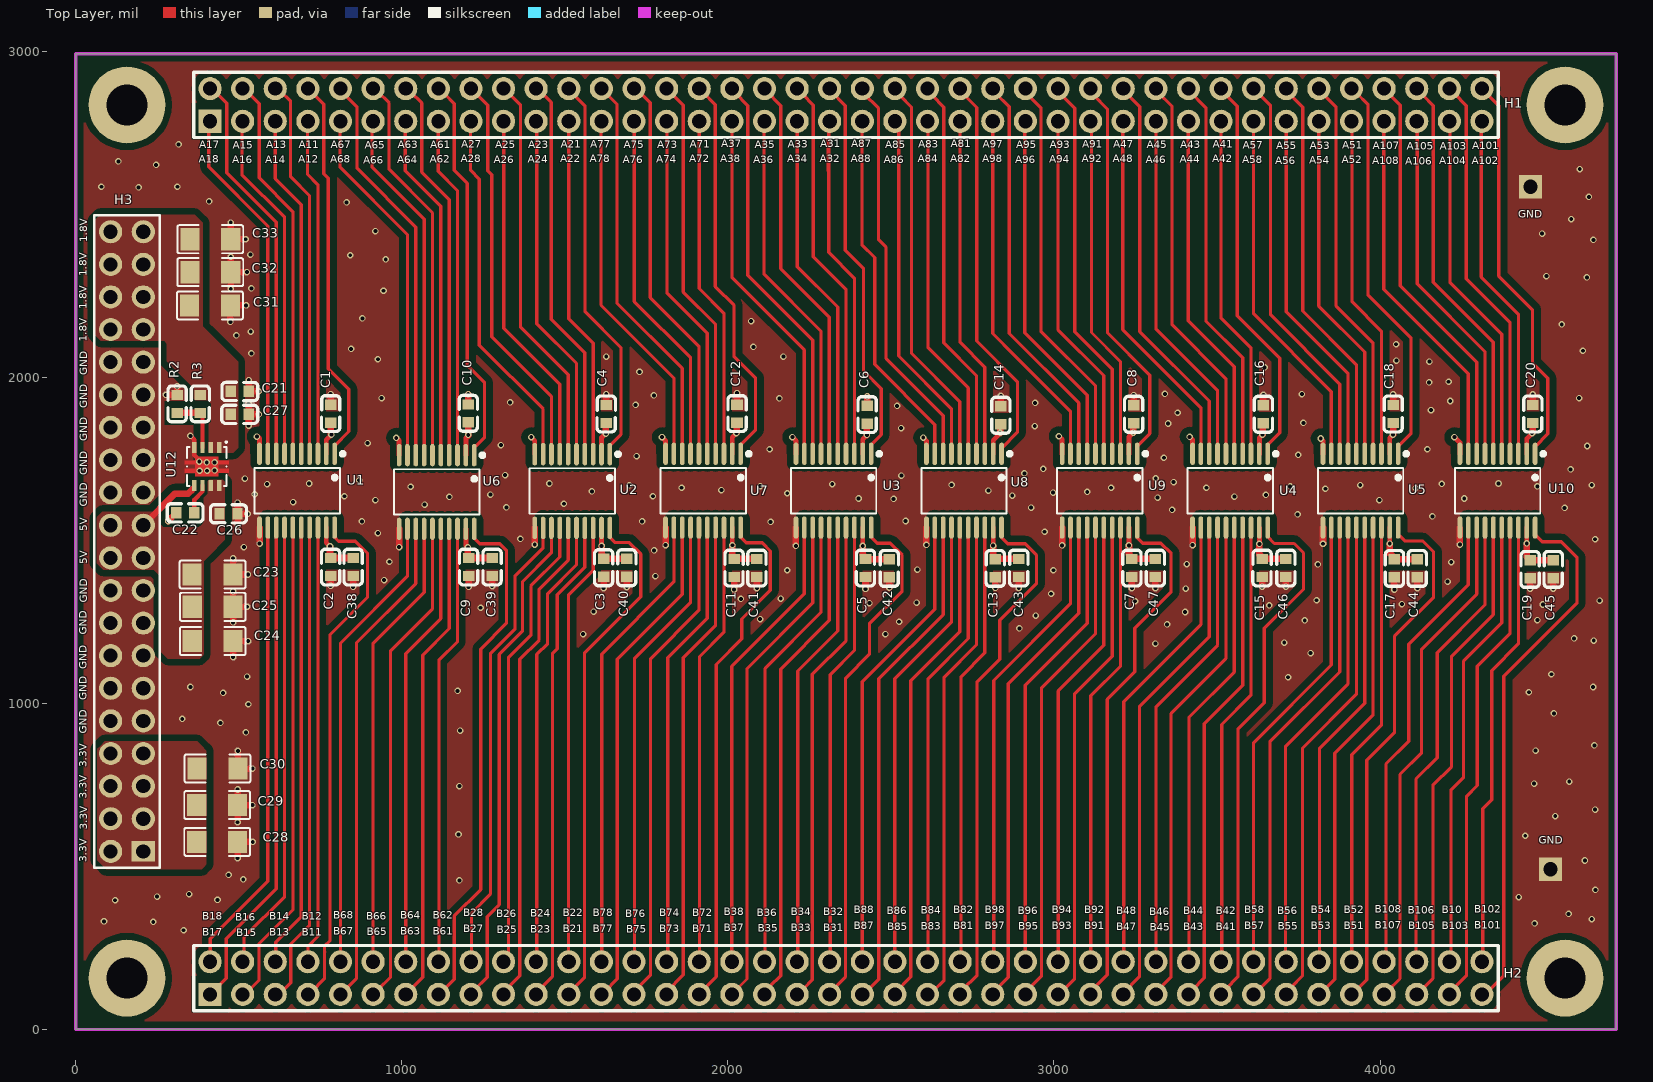
[diagram p0: Top Layer view]
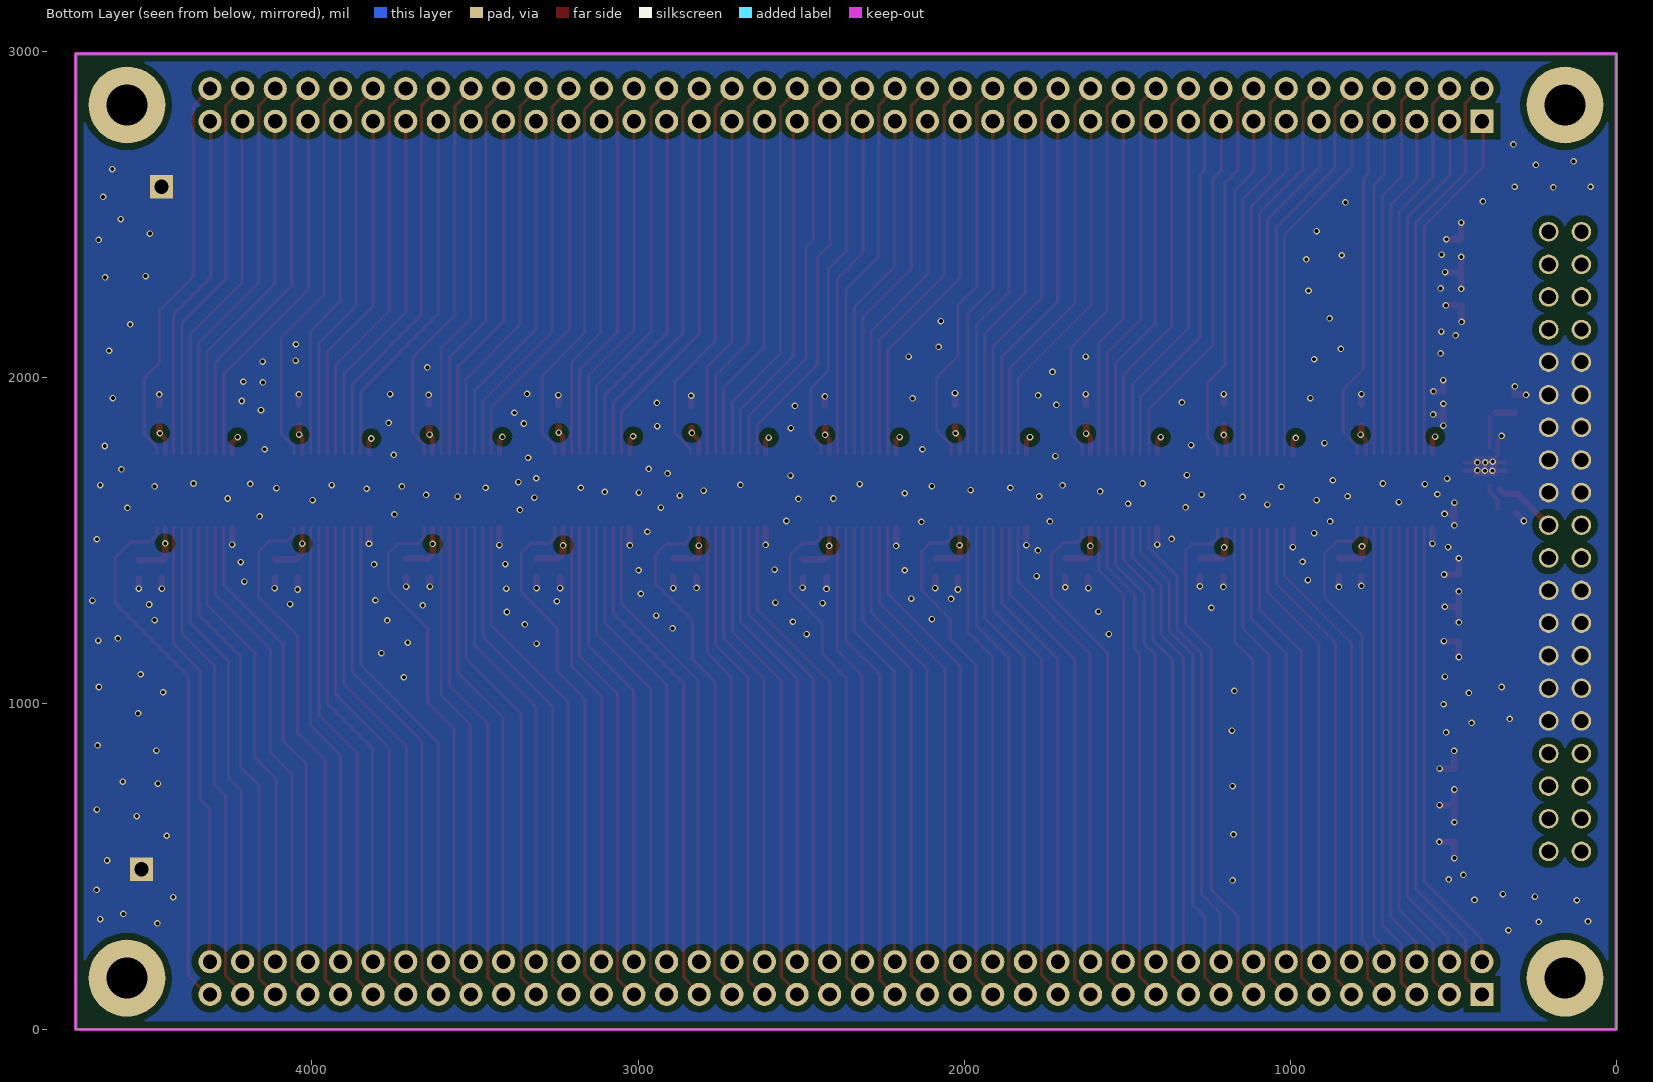
[diagram p1: Bottom Layer view, seen from below]
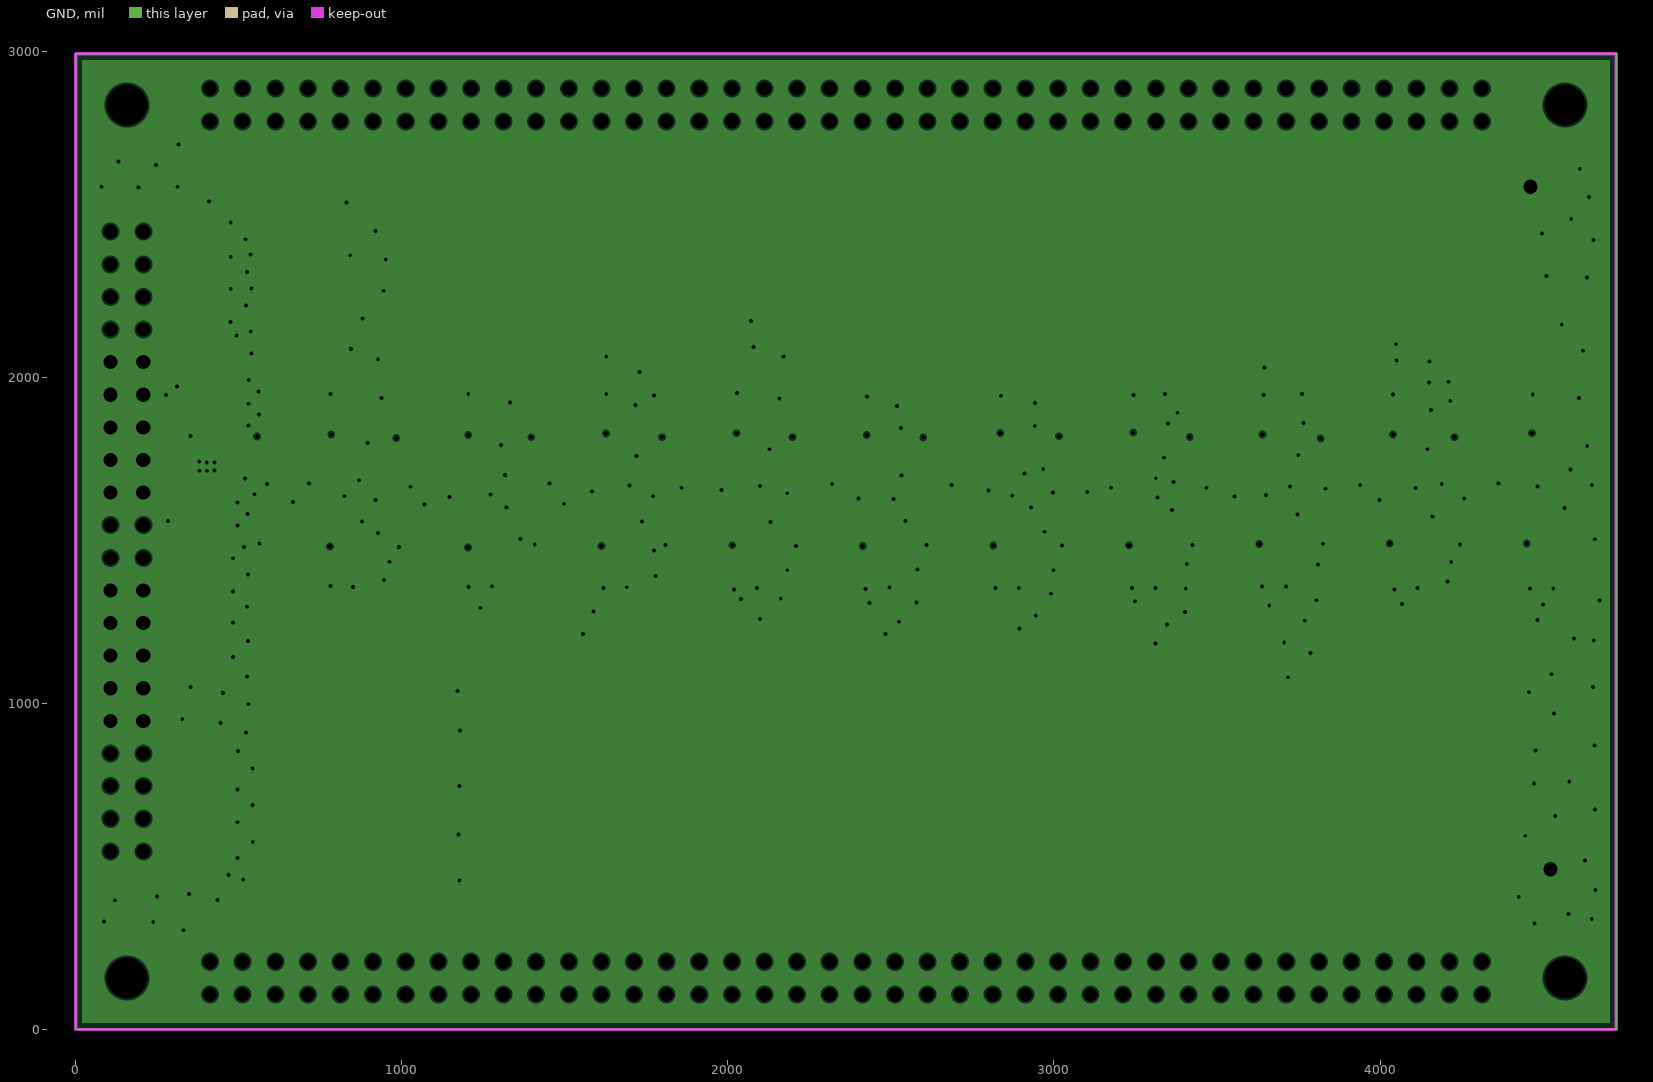
[diagram p2: GND, clearances drawn from the general rule]
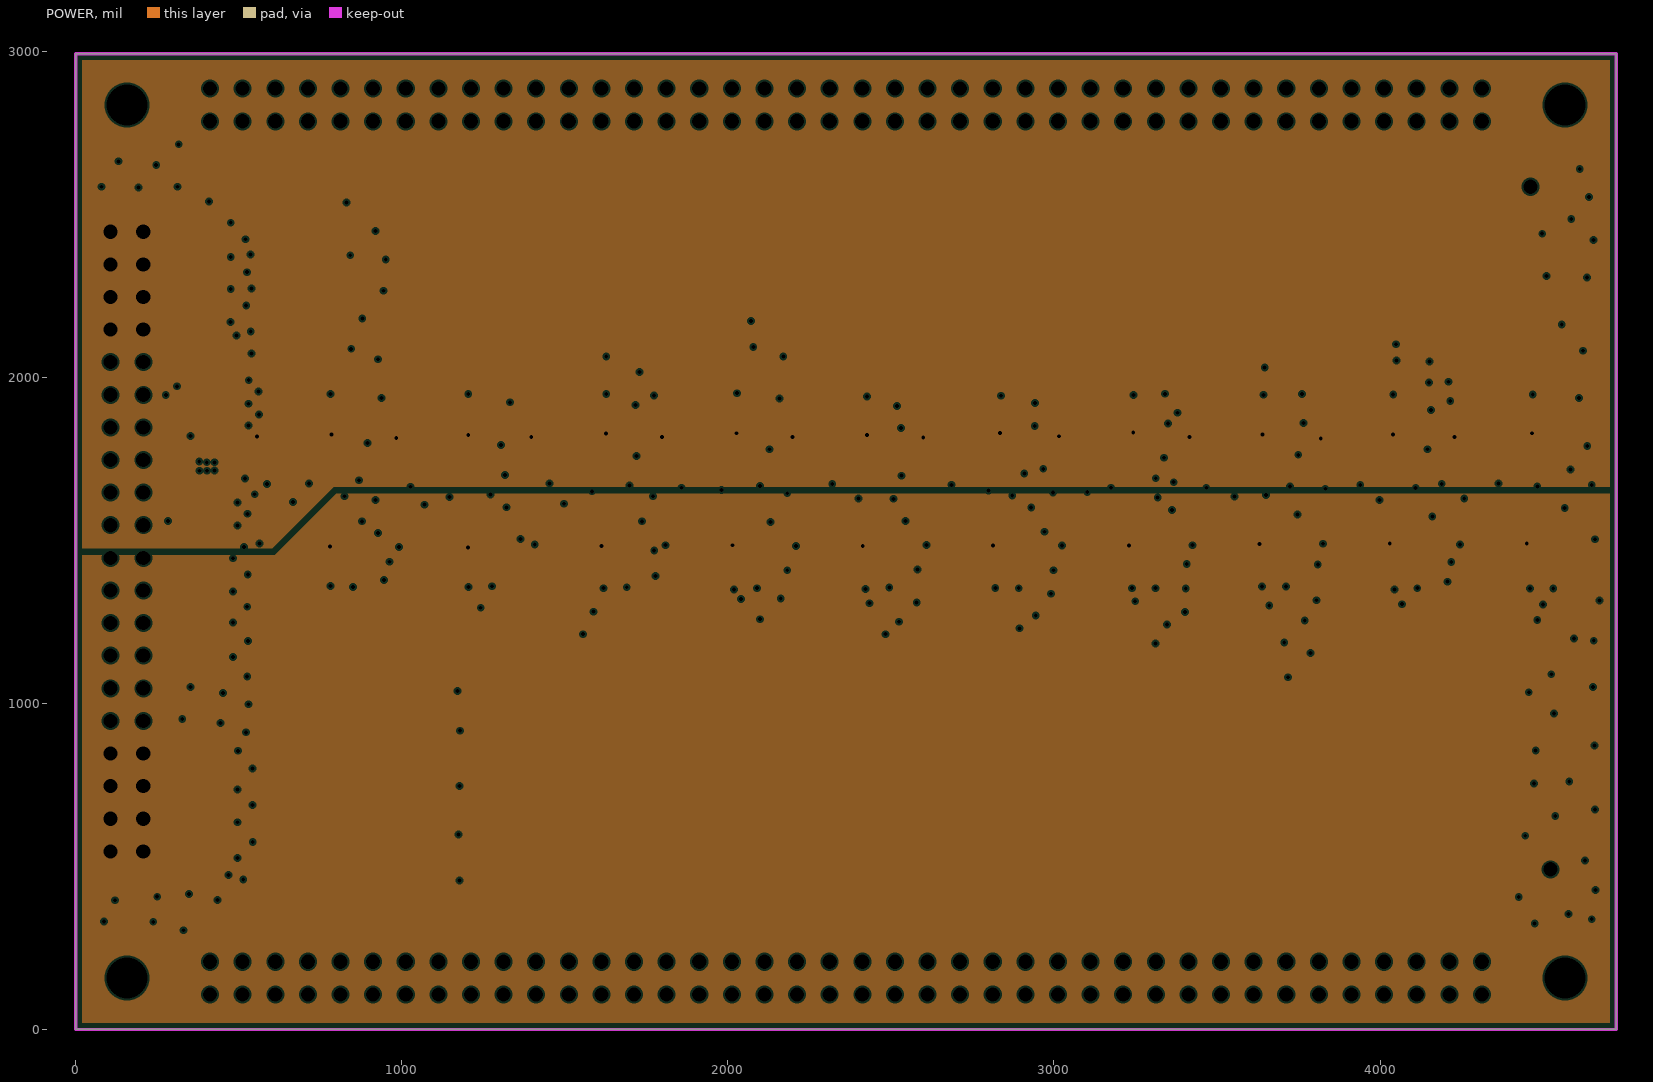
[diagram p3: POWER, clearances drawn from the general rule]
# Altium PCB MISC79033.pcbdoc (part 1 of 2)
Units mil, origin at the board's own origin, x right, y up, seen from the top; angles counter-clockwise.
Board outline 4724.41 x 2992.13 mil, 4 copper layers (Top Layer, GND, POWER, Bottom Layer); 59 components, 166 nets, 504 pads, 319 vias.

## Layer stack, top to bottom (the 12.6 mil dielectric is the usual default, probably not edited)
Top Layer: signal copper 1.4
Dielectric: core 12.6, FR-4, Dk 4.8
GND: plane copper 1.4, net GND
Dielectric: prepreg 12.6, FR-4, Dk 4.8
POWER: plane copper 1.4, net 3.3V
Dielectric: core 12.6, FR-4, Dk 4.8
Bottom Layer: signal copper 1.4

## Board outline
0,0 4724.41,0 4724.41,2992.13 0,2992.13

## Design rules (kind name [scope] priority, off if disabled: settings)
Clearance Clearance_1 [inpolygon] p1: gap=6
Clearance [All] p2: gap=6
HoleSize [All] p1: absolutevalues=TRUE maxlimit=500 minlimit=1 maxpercent=80.000 minpercent=20.000
HoleToHoleClearance [All] p1: gap=0 allowstackedmicrovias=TRUE
MinimumSolderMaskSliver [All] p1: minsoldermaskwidth=0
PlaneClearance [All] p1: clearance=6
PlaneConnect [All] p1: planeconnectstyle=Direct reliefexpansion=20 reliefentries=4 reliefconductorwidth=10 reliefairgap=10
PolygonConnect [All] p1: connectstyle=Direct reliefconductorwidth=10 reliefentries=4 polygonreliefangle="90 Angle"
RoutingVias [All] p1: holewidth=12 width=20 viastyle="Through Hole" minholewidth=12 minwidth=20 maxholewidth=12 maxwidth=20
SilkToSilkClearance [All] p1: silktosilkclearance=0
SilkscreenOverComponentPads [All] p1: minsilkscreentomaskgap=0
SolderMaskExpansion [All] p1: expansion=4
Width [All] p1: maxlimit=20 minlimit=8 preferedwidth=8 minimp=50.000000 maximp=50.000000 favimp=50.000000
21 further rules are at their usual default settings.

## Components (designator, comment, footprint, x,y, rotation, side; value= is the part's Value field where it differs from the comment)
C1 "0.1u/50V" C0603 782,1888 r270 top
C2 "0.1u/50V" C0603 782,1418 r90 top
C3 "0.1u/50V" C0603 1619,1416 r90 top
C4 "0.1u/50V" C0603 1627,1887 r270 top
C5 "0.1u/50V" C0603 2422,1415 r90 top
C6 "0.1u/50V" C0603 2427,1885 r270 top
C7 "0.1u/50V" C0603 3239,1415 r90 top
C8 "0.1u/50V" C0603 3244,1886 r270 top
C9 "0.1u/50V" C0603 1205,1418 r90 top
C10 "0.1u/50V" C0603 1204,1889 r270 top
C11 "0.1u/50V" C0603 2019,1415 r90 top
C12 "0.1u/50V" C0603 2028,1888 r270 top
C13 "0.1u/50V" C0603 2820,1414 r90 top
C14 "0.1u/50V" C0603 2837,1883 r270 top
C15 "0.1u/50V" C0603 3638,1415 r90 top
C16 "0.1u/50V" C0603 3642,1886 r270 top
C17 "0.1u/50V" C0603 4044,1414 r90 top
C18 "0.1u/50V" C0603 4040,1887 r270 top
C19 "0.1u/50V" C0603 4460,1411 r90 top
C20 "0.1u/50V" C0603 4468,1887 r270 top
C21 "4.7u/6.3v" C0603 503.26,1956.22 r180 top
C22 "10nF/50v" C0603 336,1584 r0 top
C23 "47uF/10V" C1206 420,1395 r180 top
C24 "47uF/10V" C1206 420.32,1191 r180 top
C25 "47uF/10V" C1206 420.32,1296 r180 top
C26 "1uF/50v" C0603 469,1581 r0 top
C27 "4.7u/6.3v" C0603 503,1886 r180 top
C28 "47uF/10V" C1206 434,575 r180 top
C29 "47uF/10V" C1206 434,688 r180 top
C30 "47uF/10V" C1206 435,800 r180 top
C31 "47uF/10V" C1206 411.88,2220 r180 top
C32 "47uF/10V" C1206 413,2322 r180 top
C33 "47uF/10V" C1206 413,2423 r180 top
C38 "4.7u/6.3v" C0603 851,1418 r90 top
C39 "4.7u/6.3v" C0603 1277,1418 r90 top
C40 "4.7u/6.3v" C0603 1690,1416 r90 top
C41 "4.7u/6.3v" C0603 2089,1415 r90 top
C42 "4.7u/6.3v" C0603 2495,1414 r90 top
C43 "4.7u/6.3v" C0603 2892,1415 r90 top
C44 "4.7u/6.3v" C0603 4114,1414 r90 top
C45 "4.7u/6.3v" C0603 4531,1411 r90 top
C46 "4.7u/6.3v" C0603 3711,1415 r90 top
C47 "4.7u/6.3v" C0603 3311,1415 r90 top
H1 "2.54-2*40" HDR-TH_80P-P2.54-V-M-R2-C40-S2.54 2362.2,2834.65 r0 top locked
H2 "2.54-2*40" HDR-TH_80P-P2.54-V-M-R2-C40-S2.54 2362.2,157.48 r0 top
H3 "B-2100S40P-B110" HDR-TH_40P-P2.54-V-M-R2-C20-S2.54 157.48,1496.06 r90 top locked
R2 "10k 1%" R0603 311,1918 r270 top
R3 "12.5k 1%" R0603 382,1918 r270 top
U1 "TXS0108EQPWRQ1" TSSOP-20_L6.5-W4.4-P0.65-LS6.4-BL 679,1652 r180 top
U2 "TXS0108EQPWRQ1" TSSOP-20_L6.5-W4.4-P0.65-LS6.4-BL 1523,1651 r180 top
U3 "TXS0108EQPWRQ1" TSSOP-20_L6.5-W4.4-P0.65-LS6.4-BL 2324,1652 r180 top
U4 "TXS0108EQPWRQ1" TSSOP-20_L6.5-W4.4-P0.65-LS6.4-BL 3540,1652 r180 top
U5 "TXS0108EQPWRQ1" TSSOP-20_L6.5-W4.4-P0.65-LS6.4-BL 3940,1652 r180 top
U6 "TXS0108EQPWRQ1" TSSOP-20_L6.5-W4.4-P0.65-LS6.4-BL 1107,1648 r180 top
U7 "TXS0108EQPWRQ1" TSSOP-20_L6.5-W4.4-P0.65-LS6.4-BL 1924,1652 r180 top
U8 "TXS0108EQPWRQ1" TSSOP-20_L6.5-W4.4-P0.65-LS6.4-BL 2724,1652 r180 top
U9 "TXS0108EQPWRQ1" TSSOP-20_L6.5-W4.4-P0.65-LS6.4-BL 3140,1652 r180 top
U10 "TXS0108EQPWRQ1" TSSOP-20_L6.5-W4.4-P0.65-LS6.4-BL 4360,1652 r180 top
U12 "TPS7A8001DRBR" VSON-8_L3.0-W3.0-P0.65-TL-EP 402,1726 r270 top

## Footprints (in the part's own frame and the unit in brackets; to place one, negate y for a bottom-side part, rotate by r counter-clockwise, add the part's x,y. Pads: shape width x height; smd on the part's side, far side on the other; paste and mask are expansions set on the pad)
C0603 [mm]
  rect 0.8x0.9 smd paste+0 mask+0.051: 1(-0.7,0) 2(0.7,0)
  silkscreen extent -1.41,-0.71 1.39,0.72
C1206 [mm]
  rect 1.485x1.728 smd paste-100 mask+0.051: 1(-1.593,0) 2(1.593,0)
  silkscreen extent -2.56,-1.09 2.56,1.09
HDR-TH_40P-P2.54-V-M-R2-C20-S2.54 [mm]
  rect 1.575x1.8 / inner round 1.524 / far side round 1.524 hole 1.1: 1(-24.13,-1.27)
  round 1.8 / inner round 1.524 / far side round 1.524 hole 1.1: 2(-24.13,1.27) 3(-21.59,-1.27) 4(-21.59,1.27) 5(-19.05,-1.27) 6(-19.05,1.27) 7(-16.51,-1.27) 8(-16.51,1.27) 9(-13.97,-1.27) 10(-13.97,1.27) 11(-11.43,-1.27) 12(-11.43,1.27) 13(-8.89,-1.27) 14(-8.89,1.27) 15(-6.35,-1.27) 16(-6.35,1.27) 17(-3.81,-1.27) 18(-3.81,1.27) 19(-1.27,-1.27) 20(-1.27,1.27) 21(1.27,-1.27) 22(1.27,1.27) 23(3.81,-1.27) 24(3.81,1.27) 25(6.35,-1.27) 26(6.35,1.27) 27(8.89,-1.27) 28(8.89,1.27) 29(11.43,-1.27) 30(11.43,1.27) 31(13.97,-1.27) 32(13.97,1.27) 33(16.51,-1.27) 34(16.51,1.27) 35(19.05,-1.27) 36(19.05,1.27) 37(21.59,-1.27) 38(21.59,1.27) 39(24.13,-1.27) 40(24.13,1.27)
  silkscreen extent -25.4,-2.54 25.4,2.54
HDR-TH_80P-P2.54-V-M-R2-C40-S2.54 [mm]
  rect 1.8x1.8 hole 1.1 paste+0 mask+0.051: 1(-49.53,-1.27)
  round 1.8 hole 1.1 paste+0 mask+0.051: 2(-49.53,1.27) 3(-46.99,-1.27) 4(-46.99,1.27) 5(-44.45,-1.27) 6(-44.45,1.27) 7(-41.91,-1.27) 8(-41.91,1.27) 9(-39.37,-1.27) 10(-39.37,1.27) 11(-36.83,-1.27) 12(-36.83,1.27) 13(-34.29,-1.27) 14(-34.29,1.27) 15(-31.75,-1.27) 16(-31.75,1.27) 17(-29.21,-1.27) 18(-29.21,1.27) 19(-26.67,-1.27) 20(-26.67,1.27) 21(-24.13,-1.27) 22(-24.13,1.27) 23(-21.59,-1.27) 24(-21.59,1.27) 25(-19.05,-1.27) 26(-19.05,1.27) 27(-16.51,-1.27) 28(-16.51,1.27) 29(-13.97,-1.27) 30(-13.97,1.27) 31(-11.43,-1.27) 32(-11.43,1.27) 33(-8.89,-1.27) 34(-8.89,1.27) 35(-6.35,-1.27) 36(-6.35,1.27) 37(-3.81,-1.27) 38(-3.81,1.27) 39(-1.27,-1.27) 40(-1.27,1.27) 41(1.27,-1.27) 42(1.27,1.27) 43(3.81,-1.27) 44(3.81,1.27) 45(6.35,-1.27) 46(6.35,1.27) 47(8.89,-1.27) 48(8.89,1.27) 49(11.43,-1.27) 50(11.43,1.27) 51(13.97,-1.27) 52(13.97,1.27) 53(16.51,-1.27) 54(16.51,1.27) 55(19.05,-1.27) 56(19.05,1.27) 57(21.59,-1.27) 58(21.59,1.27) 59(24.13,-1.27) 60(24.13,1.27) 61(26.67,-1.27) 62(26.67,1.27) 63(29.21,-1.27) 64(29.21,1.27) 65(31.75,-1.27) 66(31.75,1.27) 67(34.29,-1.27) 68(34.29,1.27) 69(36.83,-1.27) 70(36.83,1.27) 71(39.37,-1.27) 72(39.37,1.27) 73(41.91,-1.27) 74(41.91,1.27) 75(44.45,-1.27) 76(44.45,1.27) 77(46.99,-1.27) 78(46.99,1.27) 79(49.53,-1.27) 80(49.53,1.27)
  silkscreen extent -50.8,-2.54 50.8,2.54
R0603 [mm]
  rect 0.8x0.9 smd paste+0 mask+0.051: 1(-0.7,0) 2(0.7,0)
  silkscreen extent -1.41,-0.71 1.39,0.72
TSSOP-20_L6.5-W4.4-P0.65-LS6.4-BL [mm]
  oval 0.364x1.742 smd paste+0 mask+0.051: 1(-2.925,-2.871) 2(-2.275,-2.871) 3(-1.625,-2.871) 4(-0.975,-2.871) 5(-0.325,-2.871) 6(0.325,-2.871) 7(0.975,-2.871) 8(1.625,-2.871) 9(2.275,-2.871) 10(2.925,-2.871) 11(2.925,2.871) 12(2.275,2.871) 13(1.625,2.871) 14(0.975,2.871) 15(0.325,2.871) 16(-0.325,2.871) 17(-0.975,2.871) 18(-1.625,2.871) 19(-2.275,2.871) 20(-2.925,2.871)
  silkscreen extent -3.71,-3.02 3.33,1.77
VSON-8_L3.0-W3.0-P0.65-TL-EP [mm]
  rect 0.85x0.34 smd paste+0 mask+0.051: 1(-1.476,0.975) 2(-1.476,0.325) 3(-1.476,-0.325) 4(-1.476,-0.975) 5(1.476,-0.975) 6(1.476,-0.325) 7(1.476,0.325) 8(1.476,0.975)
  Top Layer region: -0.76,0.89 -0.47,0.89 -0.47,1.71 -0.18,1.71 -0.18,0.88 0.18,0.88 0.18,1.71 0.47,1.71 0.47,0.88 0.76,0.88 0.76,-0.89 0.47,-0.89 0.47,-1.71 0.18,-1.71 0.18,-0.89 -0.18,-0.89 -0.18,-1.71 -0.47,-1.71 -0.47,-0.89 -0.76,-0.89 -0.76,0.89
  silkscreen extent -1.96,-1.52 1.52,1.58

## Part data
C1 C2 C3 C4 C5 C6 C7 C8 C9 C10 C11 C12 C13 C14 C15 C16 C17 C18 C19 C20: library part 0.1u
C21 C27 C38 C39 C40 C41 C42 C43 C44 C45 C46 C47: library part 4.7u
C22: library part 10nF
C23 C24 C25 C28 C29 C30 C31 C32 C33: library part 4.7uF
C26: library part 1uF

## Free pads (board coordinates)
  round 236.22 hole 125.98: 0(157.48,157.48) 0(157.48,2834.65) 0(4566.93,157.48) 0(4566.93,2834.65)
  rect 70.87x70.87 hole 43.31: 1(4461,2584) 1(4523,491)

## Via types
v1: diameter 20, hole 12, Top Layer to Bottom Layer, 319 vias

## Nets (pads, with @x,y where several pads share a name; then routed paths per layer and width w, separated by ;. In a path a pad name is that pad's centre, name@x,y a point inside that pad or via, vN(x,y) a via of type N, cw(c..) or ccw(c..) an arc to the next point about the centre after c; other vN are vias at no path point)
1.8V: C1.2 C4.2 C6.2 C8.2 C10.2 C12.2 C14.2 C16.2 C18.2 C20.2 C21.2 C27.2 C31.2 C32.2 C33.2 H3.33 H3.34 H3.35 H3.36 H3.37 H3.38 H3.39 H3.40 R3.1 U1.2 U1.10 U2.2 U2.10 U3.2 U3.10 U4.2 U4.10 U5.2 U5.10 U6.2 U6.10 U7.2 U7.10 U8.2 U8.10 U9.2 U9.10 U10.2 U10.10 U12.1 U12.2 | length 1477.9
  Top Layer w13: v1@555,1820 v1@557.5,1817.5 ; v1@783,1825 v1(784,1824)
  Top Layer w14: v1@984,1813 985,1812 v1@985.5,1811.5
  Top Layer w15: v1(556,1818) 558,1818 563.84,1812.16 U1.10@563.84,1765.03 ; U1.2@768.57,1765.03 768.57,1807.57 v1@785,1824 ; v1(983,1814) v1@984,1813 ; v1@986,1812 991.84,1806.16 U6.10@991.84,1761.03 ; U6.2@1196.57,1761.03 1196.57,1813.57 1204,1821 v1(1204,1823) ; v1(1397,1816) 1407.84,1805.16 U2.10@1407.84,1764.03 ; U2.2@1612.57,1764.03 1612.57,1814.57 1626,1828 v1(1626,1827) ; v1(1798,1816) 1808.84,1805.16 U7.10@1808.84,1765.03 ; U7.2@2013.57,1765.03 2013.57,1815.57 2027,1829 v1(2026,1828) ; v1(2198,1816) 2208.84,1805.16 U3.10@2208.84,1765.03 ; U3.2@2413.57,1765.03 2413.57,1809.57 2426,1822 v1(2426,1823) ; v1(2599,1815) 2608.84,1805.16 U8.10@2608.84,1765.03 ; U8.2@2813.57,1765.03 2813.57,1806.57 2835,1828 v1(2835,1829) ; v1(3015,1819) 3024.84,1809.16 U9.10@3024.84,1765.03 ; U9.2@3229.57,1765.03 3229.57,1816.57 v1(3243,1830) ; v1(3416,1817) 3424.84,1808.16 U4.10@3424.84,1765.03 ; U4.2@3629.57,1765.03 3629.57,1813.57 3640,1824 v1(3639,1824) ; v1(3818,1812) 3824.84,1805.16 U5.10@3824.84,1765.03 ; U5.2@4029.57,1765.03 4029.57,1813.57 4040,1824 v1(4039,1824) ; v1(4228,1816) 4244.84,1799.16 U10.10@4244.84,1765.03 ; U10.2@4449.57,1765.03 4449.57,1811.57 4468,1830 v1(4466,1828)
  Top Layer w20: v1@783,1825 C1.2@783,1851 ; v1@1204,1821 C10.2@1204,1853 ; v1@1626,1828 C4.2@1626,1851 ; v1@2027,1829 C12.2@2027,1849 ; v1@2426,1822 C6.2@2426,1847 ; v1@2835,1828 C14.2@2835,1845 ; v1(3243,1830) C8.2@3243,1849 ; v1@3640,1824 C16.2@3640,1847 ; v1@4040,1824 C18.2@4040,1853 ; v1@4468,1830 C20.2@4468,1849
3.3V: C2.2 C3.2 C5.2 C7.2 C9.2 C11.2 C13.2 C15.2 C17.2 C19.2 C28.2 C29.2 C30.2 C38.2 C39.2 C40.2 C41.2 C42.2 C43.2 C44.2 C45.2 C46.2 C47.2 H3.1 H3.2 H3.3 H3.4 H3.5 H3.6 H3.7 H3.8 U1.19 U2.19 U3.19 U4.19 U5.19 U6.19 U7.19 U8.19 U9.19 U10.19 | length 1685.5
  Top Layer w15: U1.19@768.57,1538.97 768.57,1492.43 v1(780,1481) ; U6.19@1196.57,1534.97 1196.57,1484.43 v1(1203,1478) ; v1(1612.57,1482.43) U2.19@1612.57,1537.97 ; v1(2013.57,1484.57) U7.19@2013.57,1538.97 ; v1(2413.57,1482.57) U3.19@2413.57,1538.97 ; v1(2813.57,1483.43) U8.19@2813.57,1538.97 ; v1(3229.57,1484.43) U9.19@3229.57,1538.97 ; v1(3629.57,1488.57) U4.19@3629.57,1538.97 ; v1(4029.57,1489.57) U5.19@4029.57,1538.97 ; v1(4449.57,1490.43) U10.19@4449.57,1538.97
  Top Layer w20: v1@780,1479 780,1449.11 783.55,1445.55 C38.2@851,1445.55 ; v1@1202,1478 1202,1451 1207.45,1445.55 C39.2@1277,1445.55 ; v1@1613,1483 1613,1456 1625.45,1443.55 C40.2@1690,1443.55 ; v1@2014,1485 2014,1450.11 2021.55,1442.55 C41.2@2089,1442.55 ; v1@2414,1482 2414,1455 2427.45,1441.55 C42.2@2495,1441.55 ; v1@2814,1482 2814,1449 2820.44,1442.55 C43.2@2892,1442.55 ; v1@3230,1484 3230,1457 3244.44,1442.55 C47.2@3311,1442.55 ; v1@3630,1487 3630,1456 3643.44,1442.55 C46.2@3711,1442.55 ; v1@4030,1489 4030,1459 4047.44,1441.55 C44.2@4114,1441.55 ; v1@4449,1488 4449,1449.55 C19.2@4460,1438.55 ; C19.2@4455.44,1438.55 C19.2@4460,1438.55 ; C45.2@4531,1438.55 C19.2@4460,1438.55
+5V: C23.2 C24.2 C25.2 C26.1 H3.19 H3.20 H3.21 H3.22 U12.5 U12.7 U12.8 | length 196.1
  Top Layer w20: H3.21@207.48,1546.06 304.42,1643 345,1643 U12.5@358,1656
A11: H1.8 U1.1 | length 1181
  Top Layer w10: H1.8@719,2879 761,2837 761,2639 761,2637 761,2624 775,2610 775,2026 837.5,1963.5 837.5,1833.5 794.16,1790.16 U1.1@794.16,1765.03
A12: H1.7 U1.3 | length 1030.2
  Top Layer w10: H1.7@711,2782 711,2622 742.98,2590.02 U1.3@742.98,1765.03
A13: H1.6 U1.4 | length 1149
  Top Layer w10: H1.6@628,2877 659,2846 659,2614 717.39,2555.61 U1.4@717.39,1765.03
A14: H1.5 U1.5 | length 1046
  Top Layer w10: H1.5@612,2778 612,2609 691.8,2529.2 U1.5@691.8,1765.03
A15: H1.4 U1.6 | length 1170.5
  Top Layer w10: H1.4@525,2877 563,2839 563,2611 666.2,2507.8 U1.6@666.2,1765.03
A16: H1.3 U1.7 | length 1062.1
  Top Layer w10: H1.3@510,2773 510,2621 640.61,2490.39 U1.7@640.61,1765.03
A17: H1.2 U1.8 | length 1180.4
  Top Layer w10: H1.2@433,2870 463,2840 463,2627 615.02,2474.98 U1.8@615.02,1765.03
A18: H1.1 U1.9 | length 1157.9
  Top Layer w10: 408,2726 408,2654 ; H1.1@410,2775 408,2773 408,2654 ; U1.9@589.43,1765.03 589.43,2463.57 408,2645 408,2654
A21: H1.24 U2.1 | length 1181.7
  Top Layer w10: H1.24@1523,2870 1562,2831 1562,2201 1672,2091 1672,1824 1638.16,1790.16 U2.1@1638.16,1764.03
A22: H1.23 U2.3 | length 1180.3
  Top Layer w10: 1512,2632 1512,2727 ; 1512,2738.21 1512,2706 ; H1.23@1517,2784 1512,2779 1512,2706 ; U2.3@1586.98,1764.03 1586.98,2104.02 1512,2179 1512,2706
A23: H1.22 U2.4 | length 1171.3
  Top Layer w10: H1.22@1423,2878 1458.64,2842.36 1458.64,2177.36 1561.39,2074.61 U2.4@1561.39,1764.03
A24: H1.21 U2.5 | length 1064.4
  Top Layer w10: 1414,2736 1414,2724 ; H1.21@1414,2766 1414,2724 ; U2.5@1535.8,1764.03 1535.8,2042.2 1414,2164 1414,2724
A25: H1.20 U2.6 | length 1183.9
  Top Layer w10: H1.20@1327,2872 1364,2835 1364,2154 1510.2,2007.8 U2.6@1510.2,1764.03
A26: H1.19 U2.7 | length 1100.1
  Top Layer w10: 1313,2736 1313,2712 ; H1.19@1313,2769 1313,2712 ; U2.7@1484.61,1764.03 1484.61,1978.39 1313,2150 1313,2712
A27: H1.18 U2.8 | length 1204.5
  Top Layer w10: H1.18@1226,2872 1264,2834 1264,2633 1276,2621 1276,2124 1459.02,1940.98 U2.8@1459.02,1764.03
A28: H1.17 U2.9 | length 1106.5
  Top Layer w10: 1211,2733 1211,2721 ; H1.17@1212,2766 1211,2765 1211,2721 ; U2.9@1433.43,1764.03 1433.43,1902.57 1238,2098 1238,2607 1211,2634 1211,2721
A31: H1.40 U3.1 | length 1187.1
  Top Layer w10: H1.40@2317,2876 2360,2833 2360,2810 2360,2389 2416,2333 2416,2019 2470,1965 2470,1824 2439.16,1793.16 U3.1@2439.16,1765.03
A32: H1.39 U3.3 | length 1142.7
  Top Layer w10: 2308,2633 2308,2728 ; 2309,2734 2309,2714 ; H1.39@2309,2760 2309,2714 ; U3.3@2387.98,1765.03 2387.98,2304.02 2309,2383 2309,2714
A33: H1.38 U3.4 | length 1157.2
  Top Layer w10: H1.38@2229,2867 2262,2834 2262,2369 2362.39,2268.61 U3.4@2362.39,1765.03
A34: H1.37 U3.5 | length 1069.7
  Top Layer w10: 2213,2736 2213,2723 ; H1.37@2214,2770 2213,2769 2213,2723 ; U3.5@2336.8,1765.03 2336.8,2215.2 2213,2339 2213,2723
A35: H1.36 U3.6 | length 1193.4
  Top Layer w10: H1.36@2117,2878 2162,2833 2162,2333 2311.2,2183.8 U3.6@2311.2,1765.03
A36: H1.35 U3.7 | length 1094.6
  Top Layer w10: 2111,2738.21 2111,2717 ; H1.35@2116,2764 2111,2759 2111,2717 ; U3.7@2285.61,1765.03 2285.61,2141.39 2111,2316 2111,2717
A37: H1.34 U3.8 | length 1205.6
  Top Layer w10: H1.34@2022,2872 2061,2833 2061,2312 2260.02,2112.98 U3.8@2260.02,1765.03
A38: H1.33 U3.9 | length 1097.7
  Top Layer w10: 2013,2727 2013,2719 ; H1.33@2013,2763 2013,2719 ; U3.9@2234.43,1765.03 2234.43,2083.57 2013,2305 2013,2719
A41: H1.64 U4.1 | length 1197.1
  Top Layer w10: H1.64@3521,2876 3521,2872 3562,2831 3562,2188 3692,2058 3692,1830 3655.16,1793.16 U4.1@3655.16,1765.03
A42: H1.63 U4.3 | length 1040.1
  Top Layer w10: 3512,2735 3512,2727 ; H1.63@3512,2759 3512,2727 ; U4.3@3603.98,1765.03 3603.98,2090.02 3512,2182 3512,2727
A43: H1.62 U4.4 | length 1185.2
  Top Layer w10: H1.62@3409,2876 3416,2876 3465.77,2826.23 3465.77,2172.23 3578.39,2059.61 U4.4@3578.39,1765.03
A44: H1.61 U4.5 | length 1061.1
  Top Layer w10: H1.61@3414,2767 3412,2765 3412,2173 3552.8,2032.2 U4.5@3552.8,1765.03
A45: H1.60 U4.6 | length 1197
  Top Layer w10: H1.60@3317,2875 3362,2830 3362,2161 3527.2,1995.8 U4.6@3527.2,1765.03
A46: H1.59 U4.7 | length 1074.1
  Top Layer w10: H1.59@3313,2761 3313,2147 3501.61,1958.39 U4.7@3501.61,1765.03
A47: H1.58 U4.8 | length 1213
  Top Layer w10: H1.58@3220,2872 3263,2829 3263,2140 3476.02,1926.98 U4.8@3476.02,1765.03
A48: H1.57 U4.9 | length 1101.4
  Top Layer w10: 3211,2738.21 3211,2731 ; H1.57@3211,2760 3211,2731 ; U4.9@3450.43,1765.03 3450.43,1906.57 3211,2146 3211,2731
A51: H1.72 U5.1 | length 1194.5
  Top Layer w10: H1.72@3926,2873 3963,2836 3963,2251 4095,2119 4095,1828 4055.16,1788.16 U5.1@4055.16,1765.03
A52: H1.71 U5.3 | length 1039.5
  Top Layer w10: 3914,2738.21 3914,2733 ; H1.71@3914,2762 3914,2733 ; U5.3@4003.98,1765.03 4003.98,2141.02 3914,2231 3914,2733
A53: H1.70 U5.4 | length 1152.4
  Top Layer w10: H1.70@3835,2858 3865,2828 3865,2218 3978.39,2104.61 U5.4@3978.39,1765.03
A54: H1.69 U5.5 | length 1059.1
  Top Layer w10: H1.69@3814,2765 3812,2763 3812,2218 3952.8,2077.2 U5.5@3952.8,1765.03
A55: H1.68 U5.6 | length 1187.6
  Top Layer w10: H1.68@3723,2868 3763,2828 3763,2203 3927.2,2038.8 U5.6@3927.2,1765.03
A56: H1.67 U5.7 | length 1076.5
  Top Layer w10: H1.67@3712,2763 3712,2200 3901.61,2010.39 U5.7@3901.61,1765.03
A57: H1.66 U5.8 | length 1209.5
  Top Layer w10: H1.66@3626,2871 3664,2833 3664,2191 3876.02,1978.98 U5.8@3876.02,1765.03
A58: H1.65 U5.9 | length 1093.7
  Top Layer w10: H1.65@3612,2760 3612,2194 3850.43,1955.57 U5.9@3850.43,1765.03
A61: H1.16 U6.1 | length 1172.1
  Top Layer w10: H1.16@1131,2869 1161,2839 1161,2810 1161,2634 1201,2594 1201,2036 1254,1983 1254,1816 1222.16,1784.16 U6.1@1222.16,1761.03
A62: H1.15 U6.3 | length 1036.2
  Top Layer w10: 1112,2733 1112,2726 ; H1.15@1114,2765 1112,2763 1112,2726 ; U6.3@1170.98,1761.03 1170.98,2572.02 1112,2631 1112,2726
A63: H1.14 U6.4 | length 1161.6
  Top Layer w10: H1.14@1028,2874 1061,2841 1061,2629 1145.39,2544.61 U6.4@1145.39,1761.03
A64: H1.13 U6.5 | length 1060
  Top Layer w10: H1.13@1011,2776 1011,2633 1119.8,2524.2 U6.5@1119.8,1761.03
A65: H1.12 U6.6 | length 1183.2
  Top Layer w10: H1.12@927,2875 961,2841 961,2637 1094.2,2503.8 U6.6@1094.2,1761.03
A66: H1.11 U6.7 | length 1069.1
  Top Layer w10: H1.11@909,2764 909,2644 1068.61,2484.39 U6.7@1068.61,1761.03
A67: H1.10 U6.8 | length 1191
  Top Layer w10: H1.10@828,2863 863,2828 863,2640 1043.02,2459.98 U6.8@1043.02,1761.03
A68: H1.9 U6.9 | length 1108.5
  Top Layer w10: H1.9@811,2784 811,2644 1017.43,2437.57 U6.9@1017.43,1761.03
A71: H1.32 U7.1 | length 1193.6
  Top Layer w10: H1.32@1924,2873 1961,2836 1961,2808 1961,2278 2019,2220 2019,2063 2085,1997 2085,1839 2039.16,1793.16 U7.1@2039.16,1765.03
A72: H1.31 U7.3 | length 1055.7
  Top Layer w10: H1.31@1907,2769 1912,2764 1912,2720 ; 1912,2738.21 1912,2720 ; U7.3@1987.98,1765.03 1987.98,2196.02 1912,2272 1912,2720
A73: H1.30 U7.4 | length 1175.2
  Top Layer w10: H1.30@1817,2880 1863,2834 1863,2261 1962.39,2161.61 U7.4@1962.39,1765.03
A74: H1.29 U7.5 | length 1077.5
  Top Layer w10: 1813,2738.21 1813,2713 ; H1.29@1813,2766 1813,2713 ; U7.5@1936.8,1765.03 1936.8,2135.2 1813,2259 1813,2713
A75: H1.28 U7.6 | length 1196.8
  Top Layer w10: H1.28@1721,2883 1762,2842 1762,2244 1911.2,2094.8 U7.6@1911.2,1765.03
A76: H1.27 U7.7 | length 1072.5
  Top Layer w10: H1.27@1713,2766 1713,2232 1885.61,2059.39 U7.7@1885.61,1765.03
A77: H1.26 U7.8 | length 1215.6
  Top Layer w10: H1.26@1617,2880 1660,2837 1660,2227 1860.02,2026.98 U7.8@1860.02,1765.03
A78: H1.25 U7.9 | length 1120.3
  Top Layer w10: 1611,2734 1611,2715 ; H1.25@1613,2773 1611,2771 1611,2715 ; U7.9@1834.43,1765.03 1834.43,1997.57 1611,2221 1611,2715
A81: H1.48 U8.1 | length 1203
  Top Layer w10: H1.48@2713,2873 2717,2873 2763,2827 2763,2111 2888,1986 2888,1831 2839.16,1782.16 U8.1@2839.16,1765.03
A82: H1.47 U8.3 | length 1041.7
  Top Layer w10: H1.47@2709,2774 2712,2771 2712,2107 2787.98,2031.02 U8.3@2787.98,1765.03
A83: H1.46 U8.4 | length 1155.5
  Top Layer w10: H1.46@2626,2864 2662,2828 2662,2105 2762.39,2004.61 U8.4@2762.39,1765.03
A84: H1.45 U8.5 | length 1058.9
  Top Layer w10: H1.45@2612,2767 2614,2765 2614,2733 ; 2614,2738.21 2614,2733 ; U8.5@2736.8,1765.03 2736.8,1967.2 2614,2090 2614,2733
A85: H1.44 U8.6 | length 1173.9
  Top Layer w10: H1.44@2528,2863 2563,2828 2563,2073 2711.2,1924.8 U8.6@2711.2,1765.03
A86: H1.43 U8.7 | length 1063.9
  Top Layer w10: H1.43@2524,2762 2524,2065 2685.61,1903.39 U8.7@2685.61,1765.03
A87: H1.42 U8.8 | length 1207.5
  Top Layer w10: H1.42@2415,2871 2462,2824 2462,2421 2485,2398 2485,2057 2660.02,1881.98 U8.8@2660.02,1765.03
A88: H1.41 U8.9 | length 1108.7
  Top Layer w10: 2411,2738.21 2411,2723 ; H1.41@2411,2766 2411,2723 ; U8.9@2634.43,1765.03 2634.43,1854.57 2450,2039 2450,2367 2411,2406 2411,2723
A91: H1.56 U9.1 | length 1189.1
  Top Layer w10: H1.56@3120,2866 3164,2822 3164,2136 3294,2006 3294,1827 3255.16,1788.16 U9.1@3255.16,1765.03
A92: H1.55 U9.3 | length 1054.1
  Top Layer w10: H1.55@3110,2772 3115,2767 3115,2730 ; 3115,2738.21 3115,2730 ; U9.3@3203.98,1765.03 3203.98,2048.02 3115,2137 3115,2730
A93: H1.54 U9.4 | length 1168.2
  Top Layer w10: H1.54@3021,2868 3064,2825 3064,2139 3178.39,2024.61 U9.4@3178.39,1765.03
A94: H1.53 U9.5 | length 1074.2
  Top Layer w10: H1.53@3008,2770 3012,2766 3012,2729 ; 3012,2738.21 3012,2729 ; U9.5@3152.8,1765.03 3152.8,2005.2 3012,2146 3012,2729
A95: H1.52 U9.6 | length 1189.6
  Top Layer w10: H1.52@2918,2868 2960,2826 2960,2141 3127.2,1973.8 U9.6@3127.2,1765.03
A96: H1.51 U9.7 | length 1102.2
  Top Layer w10: H1.51@2906,2774 2910,2770 2910,2726 ; 2910,2738.21 2910,2726 ; U9.7@3101.61,1765.03 3101.61,1944.39 2910,2136 2910,2726
A97: H1.50 U9.8 | length 1214.4
  Top Layer w10: H1.50@2819,2873 2863,2829 2863,2134 3076.02,1920.98 U9.8@3076.02,1765.03
A98: H1.49 U9.9 | length 1169.4
  Top Layer w10: H1.49@2805,2772 2812,2765 2812,2134 2889,2057 ; 2846,2100 2889,2057 ; U9.9@3050.43,1765.03 3050.43,1895.57 2889,2057
A101: H1.80 U10.1 | length 1194.7
  Top Layer w10: H1.80@4329,2867 4364,2832 4364,2809 4364,2310 4467,2207 4467,2044 4514,1997 4514,1826 4475.16,1787.16 U10.1@4475.16,1765.03
A102: H1.79 U10.3 | length 1051.2
  Top Layer w10: 4310,2735 4310,2728 ; H1.79@4310,2762 4310,2728 ; U10.3@4423.98,1765.03 4423.98,2193.02 4310,2307 4310,2728
A103: H1.78 U10.4 | length 1176
  Top Layer w10: H1.78@4227,2870 4264,2833 4264,2302 4398.39,2167.61 U10.4@4398.39,1765.03
A104: H1.77 U10.5 | length 1068.2
  Top Layer w10: H1.77@4213,2767 4214,2766 4214,2291 4372.8,2132.2 U10.5@4372.8,1765.03
A105: H1.76 U10.6 | length 1190.9
  Top Layer w10: H1.76@4130,2866 4163,2833 4163,2291 4347.2,2106.8 U10.6@4347.2,1765.03
A106: H1.75 U10.7 | length 1078
  Top Layer w10: H1.75@4114,2757 4114,2286 4321.61,2078.39 U10.7@4321.61,1765.03
A107: H1.74 U10.8 | length 1218.2
  Top Layer w10: H1.74@4025,2871 4062,2834 4062,2280 4296.02,2045.98 U10.8@4296.02,1765.03
A108: H1.73 U10.9 | length 1104.4
  Top Layer w10: H1.73@4011,2762 4011,2270 4270.43,2010.57 U10.9@4270.43,1765.03
B11: H2.7 U1.20 | length 1568.6
  Top Layer w10: H2.7@722,114 763,155 763,237 763.5,237.5 ; 763,238 763,255 780,272 780,1210 895,1325 895,1460 858,1497 806,1497 794.16,1508.84 U1.20@794.16,1538.97
B12: H2.8 U1.18 | length 1344.2
  Top Layer w10: H2.8@712.2,207.48 712.2,254.2 743,285 743,1374 U1.18@742.98,1538.97
B13: H2.5 U1.17 | length 1463.6
  Top Layer w10: H2.5@629,112 660,143 660,234 660,236 660,262 717.39,319.39 U1.17@717.39,1538.97
B14: H2.6 U1.16 | length 1364.3
  Top Layer w10: H2.6@614,218 614,267 ; 614,256 614,267 ; 691.8,1337 U1.16@691.8,1538.97 ; 692,1337 692,345 614,267
B15: H2.3 U1.15 | length 1491.5
  Top Layer w10: H2.3@520,108 562,150 562,262 666.2,366.2 U1.15@666.2,1538.97
B16: H2.4 U1.14 | length 1372.6
  Top Layer w10: H2.4@516,218 516,282 640.61,406.61 U1.14@640.61,1538.97
B17: H2.1 U1.13 | length 1494.9
  Top Layer w10: H2.1@427,122 462,157 462,278 615.02,431.02 U1.13@615.02,1538.97
B18: H2.2 U1.12 | length 1405.5
  Top Layer w10: 413,257 413,267 ; H2.2@414,217 413,218 413,267 ; U1.12@589.43,1538.97 589.43,454.43 413,278 413,267
B21: H2.23 U2.20 | length 1573.3
  Top Layer w10: H2.23@1520,118 1560,158 1560,1154 1733,1327 1733,1458 1698,1493 1654,1493 1638.16,1508.84 U2.20@1638.16,1537.97
B22: H2.24 U2.18 | length 1378.4
  Top Layer w10: H2.24@1511,226 1511,295 ; 1511,260 1511,295 ; U2.18@1586.98,1537.97 1586.98,1407.98 1511,1332 1511,295
B23: H2.21 U2.17 | length 1472.3
  Top Layer w10: H2.21@1423,123 1462,162 1462,1152 1477,1167 1477,1333 1561.39,1417.39 U2.17@1561.39,1537.97